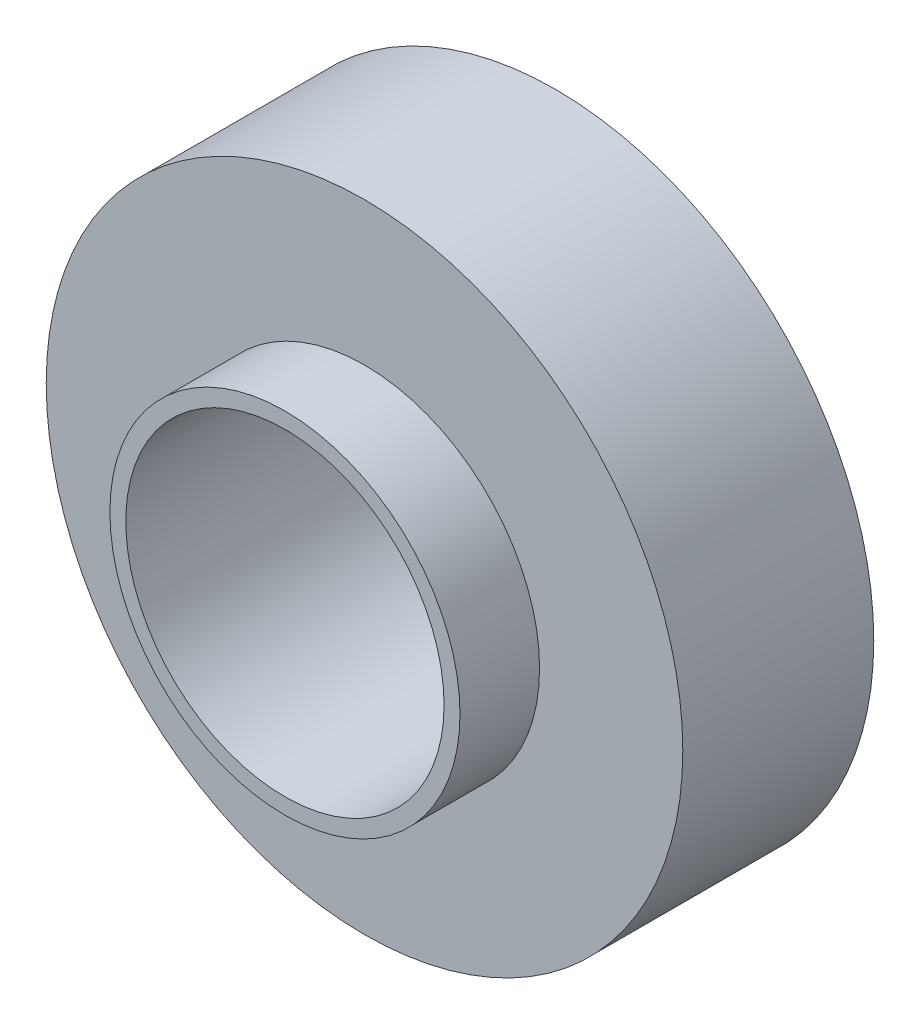
from build123d import *

# Parameters (mm, degrees)
SKETCH1_R           = 20
SKETCH1_R_2         = 10
BOSS_EXTRUDE1_DEPTH = 12
SKETCH2_R           = 11
SKETCH2_R_2         = 10
BOSS_EXTRUDE2_DEPTH = 5


with BuildPart() as part:
    # Sketch1 → Boss-Extrude1 (new body)
    with BuildSketch(Plane.XY):
        Circle(SKETCH1_R)
        Circle(SKETCH1_R_2, mode=Mode.SUBTRACT)
    extrude(amount=BOSS_EXTRUDE1_DEPTH)

    # Sketch2 → Boss-Extrude2 (add)
    with BuildSketch(Plane.XY.offset(12)):
        Circle(SKETCH2_R)
        Circle(SKETCH2_R_2, mode=Mode.SUBTRACT)
    extrude(amount=BOSS_EXTRUDE2_DEPTH)


solid = part.part
